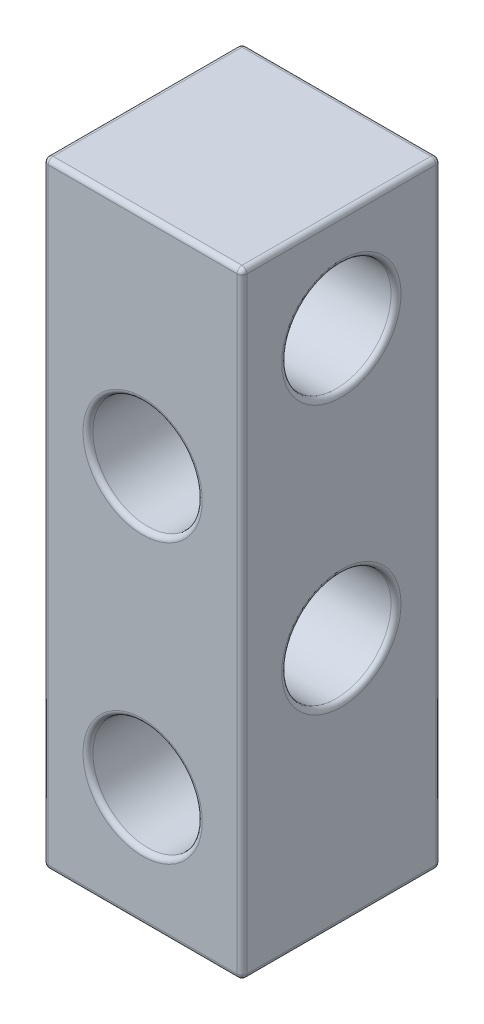
SolidWorks part; units mm, degrees
material "ABS PC"
ref_plane "Front Plane" through (0, 0, 0) normal (0, 0, 1) x (1, 0, 0)
ref_plane "Top Plane" through (0, 0, 0) normal (0, 1, 0) x (1, 0, 0)
ref_plane "Right Plane" through (0, 0, 0) normal (1, 0, 0) x (0, 0, -1)
sketch "Sketch1" plane through (0, 0, 0) normal (0, 0, 1) x (1, 0, 0)
  line L1 (10, -31) -> (-10, -31)
  line L2 (10, -31) -> (10, 31)
  line L3 (10, 31) -> (-10, 31)
  line L4 (-10, -31) -> (-10, 31)
  line L5 (10, -31) -> (-10, 31) construction
  line L6 (10, 31) -> (-10, -31) construction
  circle A0 centre (0, -19) radius 5.5
  circle A1 centre (0, 9) radius 5.5
  point P0 (0, 0)
  dimension "D3" = 28
  dimension "D4" = 12
  dimension "D5" = 11
  dimension "D1" = 20
  dimension "D2" = 62
extrude "Boss-Extrude1" add sketch "Sketch1" along normal mid plane 20
sketch "Sketch2" plane through (10, 0, 0) normal (1, 0, 0) x (0, 0, -1)
  line L0 (-10, 31) -> (10, 31) construction
  circle A0 centre (0, 21) radius 5.5
  circle A1 centre (0, -6) radius 5.5
  point P4 (0, 31)
  dimension "D1" = 10
  dimension "D2" = 11
  dimension "D3" = 27
extrude "Cut-Extrude1" cut sketch "Sketch2" against normal blind 20
fillet "Fillet1" radius 0.5 20 edges at (-10, -31, 0) (-10, 21, -5.5) (-10, -6, -5.5) (5.5, 9, -10) (0, -31, -10) (-10, 0, -10) (5.5, -19, -10) (10, -31, 0) (10, 0, -10) (10, 21, -5.5) (10, -6, -5.5) (5.5, 9, 10) (10, 0, 10) (0, -31, 10) (-10, 0, 10) (5.5, -19, 10) (10, 31, 0) (0, 31, 10) (-10, 31, 0) (0, 31, -10)
